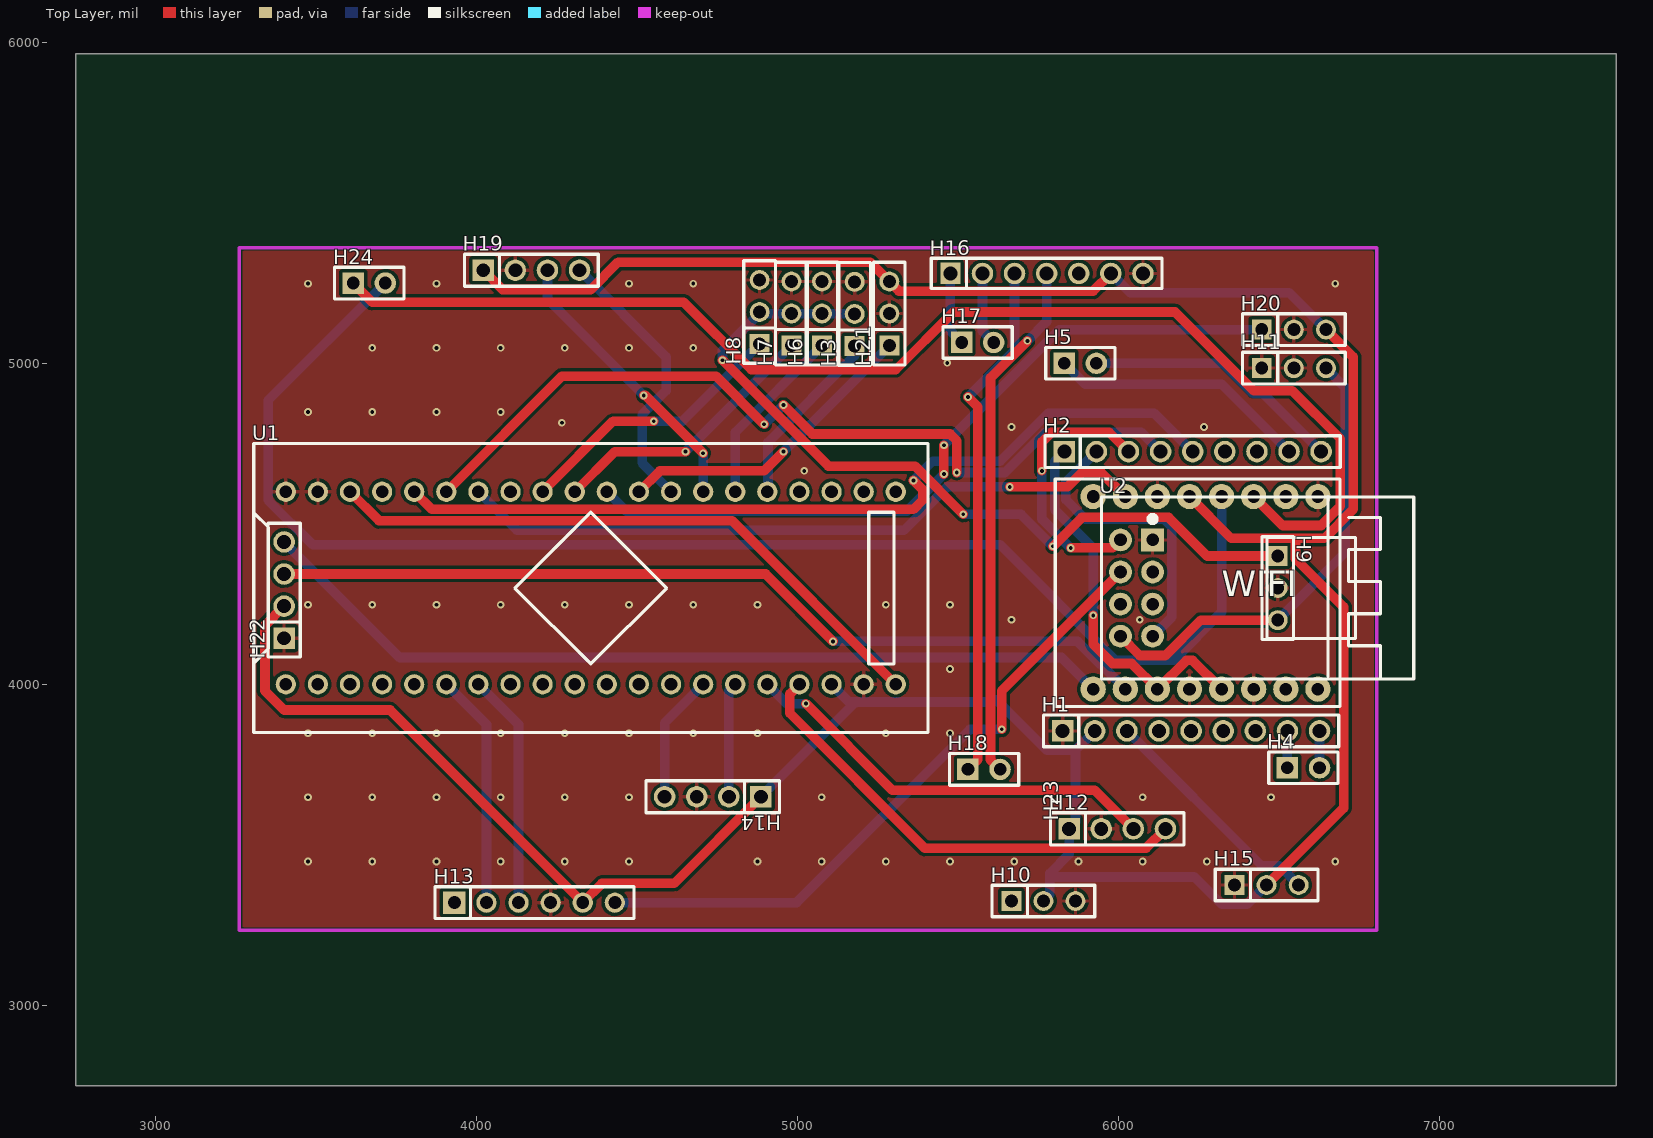
[diagram p0: Top Layer view]
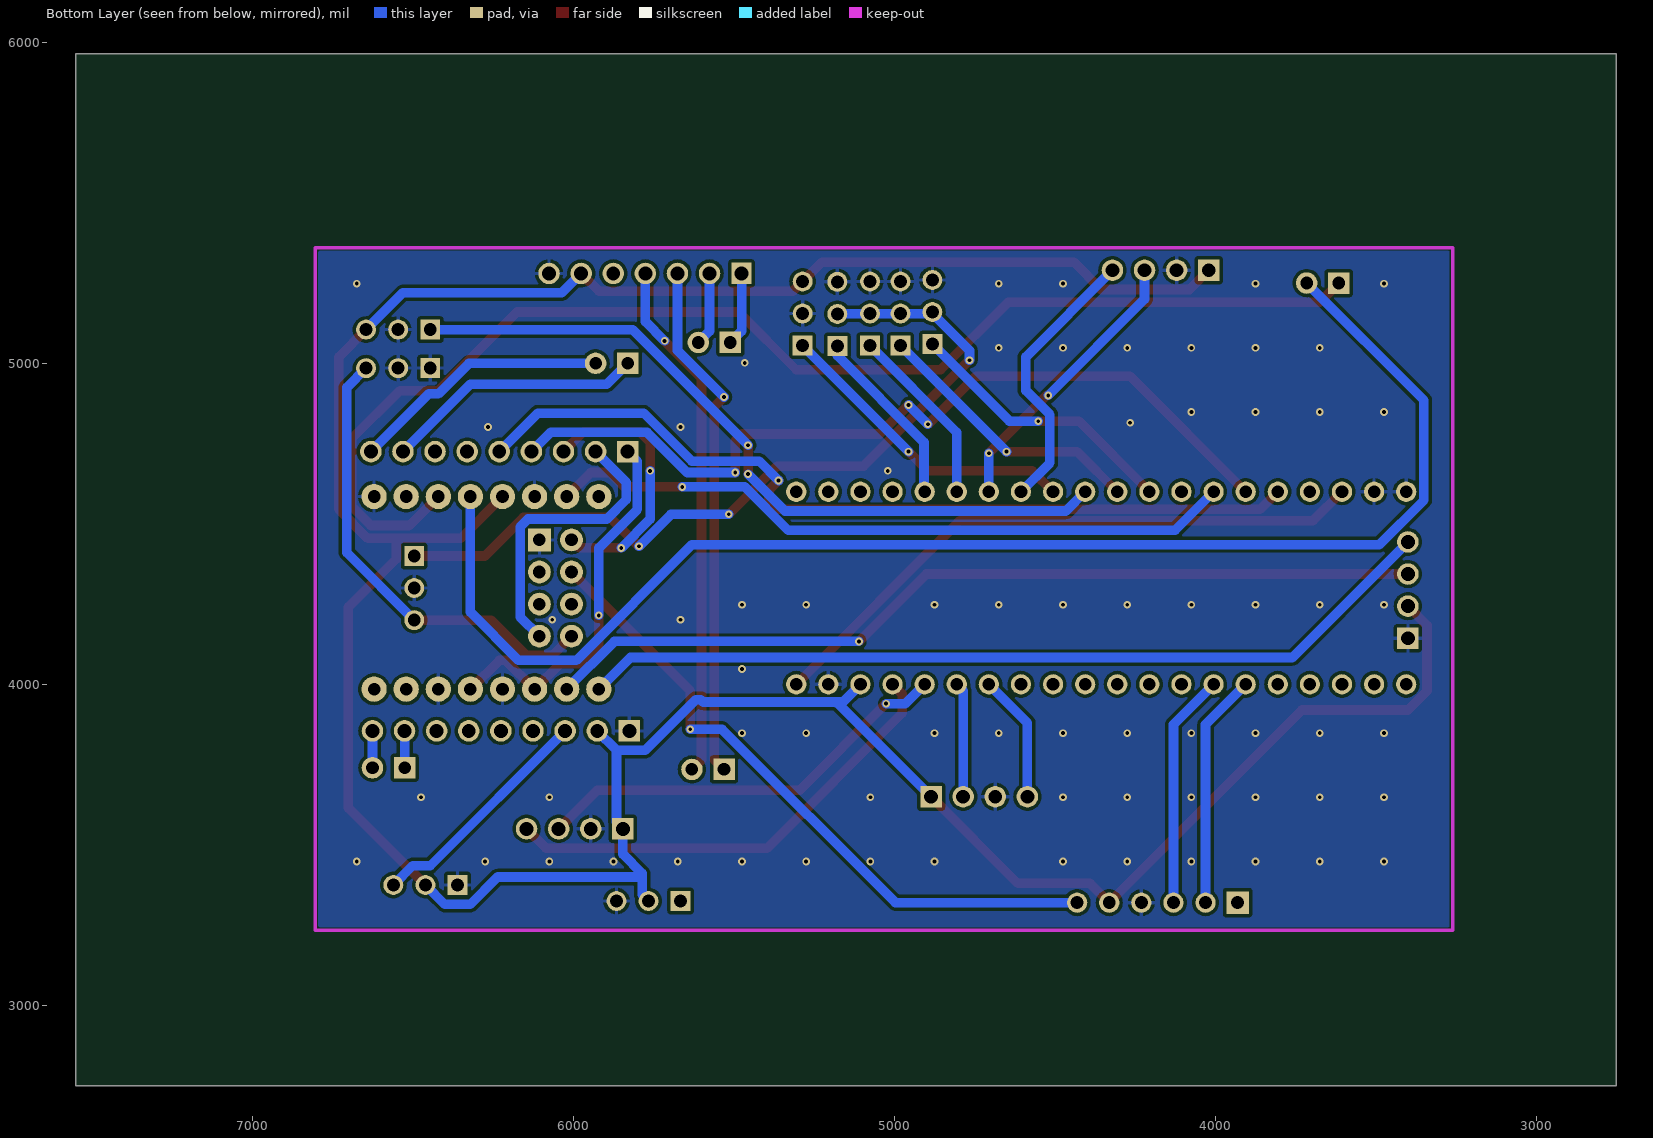
[diagram p1: Bottom Layer view, seen from below]
# Altium PCB MISC49865.pcbdoc
Units mil, origin at the board's own origin, x right, y up, seen from the top; angles counter-clockwise.
Board outline 4800 x 3215 mil, 2 copper layers (Top Layer, Bottom Layer), stack 62.206 mil thick; 26 components, 71 nets, 151 pads, 90 vias.

## Layer stack, top to bottom
Top Solder Mask Layer: solder mask 0.394, Dk 3.3
Top Layer: signal copper 1.379
Dielectric1: surface 59.449, FR4, Dk 4.5
Bottom Layer: signal copper 1.378
Bottom Solder Mask Layer: solder mask 0.394, Dk 3.3

## Board outline
7550,2750 2750,2750 2750,5965 7550,5965

## Design rules (kind name [scope] priority, off if disabled: settings)
BoardOutlineClearance copperThickness2oz_1 [All] p2 off: genericclearance=7.99 ignorepadtopadclearanceinfootprint=FALSE except(0: Arc-SplitContinuation Track-SplitContinuation SMDPad-SplitContinuation THPad-SplitContinuation Via-SplitContinuation Fill-SplitContinuation Region-SplitContinuation Poly-SplitContinuation Text-SplitContinuation Hole-SplitContinuation; 5.98: Arc-CutoutEdge SMDPad-CutoutEdge THPad-CutoutEdge Via-CutoutEdge Fill-CutoutEdge Region-CutoutEdge Text-CutoutEdge; 6.93: Hole-OutlineEdge Hole-CutoutEdge; 10: Poly-OutlineEdge Poly-CutoutEdge; 11.81: Arc-OutlineEdge Track-OutlineEdge SMDPad-OutlineEdge THPad-OutlineEdge Via-OutlineEdge Fill-OutlineEdge Region-OutlineEdge Text-OutlineEdge Track-CutoutEdge)
BoardOutlineClearance copperThickness1oz_1 [All] p4: genericclearance=4.02 ignorepadtopadclearanceinfootprint=FALSE except(0: Arc-SplitContinuation Track-SplitContinuation SMDPad-SplitContinuation THPad-SplitContinuation Via-SplitContinuation Fill-SplitContinuation Region-SplitContinuation Poly-SplitContinuation Text-SplitContinuation Hole-SplitContinuation; 6: SMDPad-CutoutEdge THPad-CutoutEdge Via-CutoutEdge Fill-CutoutEdge Region-CutoutEdge Text-CutoutEdge; 6.93: Hole-OutlineEdge Hole-CutoutEdge; 10: Poly-OutlineEdge Poly-CutoutEdge; 11.8: Arc-OutlineEdge Track-OutlineEdge SMDPad-OutlineEdge THPad-OutlineEdge Via-OutlineEdge Fill-OutlineEdge Region-OutlineEdge Text-OutlineEdge; 11.81: Arc-CutoutEdge Track-CutoutEdge)
Clearance copperThickness2oz [All] p1 off: gap=7.99 ignorepadtopadclearanceinfootprint=FALSE except(5.98: SMDPad-Track SMDPad-SMDPad THPad-Track SMDPad-THPad THPad-THPad Track-Via SMDPad-Via THPad-Via Via-Via Fill-Track Region-Track Fill-SMDPad Region-SMDPad Fill-THPad Region-THPad Fill-Via Region-Via Fill-Fill Fill-Region Region-Region Arc-Track Arc-SMDPad Arc-THPad Arc-Via Fill-Arc Region-Arc Arc-Arc Text-Track SMDPad-Text Text-THPad Text-Via Fill-Text Region-Text Arc-Text Text-Text; 6.93: Hole-Track Hole-SMDPad Hole-THPad Hole-Via Fill-Hole Region-Hole Hole-Arc Hole-Text; 10: Poly-Track Poly-SMDPad Poly-THPad Poly-Via Poly-Fill Poly-Region Poly-Poly Poly-Arc Poly-Text Poly-Hole)
Clearance copperThickness1oz [All] p3: gap=4.02 ignorepadtopadclearanceinfootprint=FALSE except(5.98: SMDPad-Track SMDPad-SMDPad THPad-Track SMDPad-THPad THPad-THPad Track-Via SMDPad-Via THPad-Via Via-Via Fill-Track Region-Track Fill-SMDPad Region-SMDPad Fill-THPad Region-THPad Fill-Via Region-Via Fill-Fill Fill-Region Region-Region; 6: Arc-Track Arc-SMDPad Arc-THPad Arc-Via Fill-Arc Region-Arc Arc-Arc Text-Track SMDPad-Text Text-THPad Text-Via Fill-Text Region-Text Arc-Text Text-Text; 6.93: Hole-Track Hole-SMDPad Hole-THPad Hole-Via Fill-Hole Region-Hole Hole-Arc Hole-Text; 10: Poly-Track Poly-SMDPad Poly-THPad Poly-Via Poly-Fill Poly-Region Poly-Poly Poly-Arc Poly-Text Poly-Hole)
DiffPairsRouting differentialPair [All] p1: maxlimit=6 minlimit=6 mostfreqgap=6 toplayer_minwidth=5 toplayer_prefwidth=10 toplayer_maxwidth=100 toplayer_mingap=6 toplayer_prefgap=6 toplayer_maxgap=6 bottomlayer_minwidth=5 bottomlayer_prefwidth=10 bottomlayer_maxwidth=100 bottomlayer_mingap=6 bottomlayer_prefgap=6 bottomlayer_maxgap=6 maxuncoupledlength=10
HoleToHoleClearance otherClearance [All] p1: gap=11.81 allowstackedmicrovias=TRUE
Length netLength [All] p1: minlimit=0 maxlimit=0
MatchedLengths netLengthTolerance [All] p1: tolerance=1000
PasteMaskExpansion pasteMaskExpansion [All] p1: expansion=0
PlaneConnect innerPlane [All] p1: planeconnectstyle=Relief reliefexpansion=20 reliefentries=4 reliefconductorwidth=10 reliefairgap=10
PolygonConnect copperRegion [All] p1: connectstyle=Relief reliefconductorwidth=10 reliefentries=4 polygonreliefangle="90 Angle" airgapwidth=10 via.connectstyle=Relief via.reliefconductorwidth=10 via.reliefentries=4 via.polygonreliefangle="90 Angle" via.airgapwidth=10
RoutingVias viaSize [All] p1: holewidth=12.01 width=24.02 viastyle="Through Hole" minholewidth=11.81 minwidth=19.68 maxholewidth=248.03 maxwidth=393.7
SolderMaskExpansion solderMaskExpansion [IsVia] p1: expansion=-1000 istentingtop=TRUE
SolderMaskExpansion solderMaskExpansion [All] p2: expansion=2 istentingtop=FALSE
Width copperThickness2oz_2 [All] p1 off: maxlimit=100 minlimit=8 preferedwidth=10
Width copperThickness1oz_2 [All] p2: maxlimit=10 minlimit=10 preferedwidth=10 toplayer_minwidth=30 toplayer_maxwidth=100 toplayer_prefwidth=30 bottomlayer_minwidth=30 bottomlayer_maxwidth=100 bottomlayer_prefwidth=30

## Components (designator, comment, footprint, x,y, rotation, side; value= is the part's Value field where it differs from the comment)
H1 "" HDR-TH_9P-P2.54-V-F-1 6225,3855 r0 top
H2 "" HDR-TH_9P-P2.54-V-F-1 6230,4725 r0 top
H3 "" HDR-TH_3P-P2.54-V-F 5176.94,5153.94 r90 top
H4 "" HDR-TH_2P-P2.54-V-F 6575,3740 r0 top
H5 "" HDR-TH_2P-P2.54-V-F 5880,5000 r0 top
H6 "" HDR-TH_3P-P2.54-V-F 5075,5155 r90 top
H7 "" HDR-TH_3P-P2.54-V-F 4980,5155 r90 top
H8 "" HDR-TH_3P-P2.54-V-F 4880.94,5159.77 r90 top
H9 "" HDR-TH_3P-P2.54-V-F 6495,4300 r270 top
H10 "" HDR-TH_3P-P2.54-V-F 5765,3325 r0 top
H11 "" HDR-TH_3P-P2.54-V-F 6545,4985 r0 top
H12 "" HDR-TH_4P-P2.54-V-F 5995,3550 r0 top
H13 "" HDR-TH_6P-P2.54-V-F 4180,3320 r0 top
H14 "" HDR-TH_4P-P2.54-V-F 4735,3650 r180 top
H15 "" HDR-TH_3P-P2.54-V-F 6460,3375 r0 top
H16 "" HDR-TH_7P-P2.54-V-F 5775,5280 r0 top
H17 "" HDR-TH_2P-P2.54-V-F 5560,5065 r0 top
H18 "" HDR-TH_2P-P2.54-V-F 5580,3735 r0 top
H19 "" HDR-TH_4P-P2.54-V-F 4170,5290 r0 top
H20 "" HDR-TH_3P-P2.54-V-F 6545,5105 r0 top
H21 "" HDR-TH_3P-P2.54-V-F 5285,5155 r90 top
H22 "" HDR-TH_4P-P2.54-V-F 3399.74,4293.7 r90 top
H23 "" ESP32C3MINI 5920,3985 r90 top
H24 "" HDR-TH_2P-P2.54-V-F 3665,5250 r0 top
U1 "STM32F103C8T6-Card" CONN-TH_L53.3-W22.9_STM32F103C8T6-CARD 4355,4300 r0 top
U2 "Ai-Thinker ESP-01S ESP8266" WIFIM-TH_8P-L24.7-W14.4-P2.54 6055,4300 r0 top

## Footprints (in the part's own frame and the unit in brackets; to place one, negate y for a bottom-side part, rotate by r counter-clockwise, add the part's x,y. Pads: shape width x height; smd on the part's side, far side on the other; paste and mask are expansions set on the pad)
CONN-TH_L53.3-W22.9_STM32F103C8T6-CARD [mm]
  round 1.6 hole 1: 1(-24.13,-7.62) 2(-21.59,-7.62) 3(-19.05,-7.62) 4(-16.51,-7.62) 5(-13.97,-7.62) 6(-11.43,-7.62) 7(-8.89,-7.62) 8(-6.35,-7.62) 9(-3.81,-7.62) 10(-1.27,-7.62) 11(1.27,-7.62) 12(3.81,-7.62) 13(6.35,-7.62) 14(8.89,-7.62) 15(11.43,-7.62) 16(13.97,-7.62) 17(16.51,-7.62) 18(19.05,-7.62) 19(21.59,-7.62) 20(24.13,-7.62) 21(24.13,7.62) 22(21.59,7.62) 23(19.05,7.62) 24(16.51,7.62) 25(13.97,7.62) 26(11.43,7.62) 27(8.89,7.62) 28(6.35,7.62) 29(3.81,7.62) 30(1.27,7.62) 31(-1.27,7.62) 32(-3.81,7.62) 33(-6.35,7.62) 34(-8.89,7.62) 35(-11.43,7.62) 36(-13.97,7.62) 37(-16.51,7.62) 38(-19.05,7.62) 39(-21.59,7.62) 40(-24.13,7.62)
  silkscreen extent -26.67,-11.43 26.67,11.43
ESP32C3MINI [mm]
  round 2 hole 1: 1(0,0) 2(0,-2.54) 3(0,-5.08) 4(0,-7.62) 5(0,-10.16) 6(0,-12.7) 7(0,-15.24) 8(0,-17.78) 9(15.24,-17.78) 10(15.24,-15.24) 11(15.24,-12.7) 12(15.24,-10.16) 13(15.24,-7.62) 14(15.24,-5.08) 15(15.24,-2.54) 16(15.24,0)
  silkscreen extent -1.38,-20.75 16.62,3
HDR-TH_2P-P2.54-V-F [mm]
  rect 1.7x1.7 hole 1: 1(-1.27,0)
  round 1.7 hole 1: 2(1.27,0)
  silkscreen extent -2.74,-1.25 2.74,1.25
HDR-TH_3P-P2.54-V-F [mil]
  rect 62x62 hole 40.16: 1(-100,0)
  round 62 hole 40.16: 2(0,0) 3(100,0)
  silkscreen extent -160,-49 160,49
HDR-TH_4P-P2.54-V-F [mm]
  rect 1.7x1.7 hole 1.1: 1(-3.81,0)
  round 1.7 hole 1.1: 2(-1.27,0) 3(1.27,0) 4(3.81,0)
  silkscreen extent -5.29,-1.27 5.29,1.27
HDR-TH_6P-P2.54-V-F [mm]
  rect 1.8x1.8 hole 1.02: 1(-6.35,0)
  round 1.6 hole 1.02: 2(-3.81,0) 3(-1.27,0) 4(1.27,0) 5(3.81,0) 6(6.35,0)
  silkscreen extent -7.87,-1.25 7.87,1.25
HDR-TH_7P-P2.54-V-F [mm]
  rect 1.575x1.7 hole 1.1: 1(-7.62,0)
  round 1.7 hole 1.1: 2(-5.08,0) 3(-2.54,0) 4(0,0) 5(2.54,0) 6(5.08,0) 7(7.62,0)
  silkscreen extent -9.13,-1.2 9.13,1.2
HDR-TH_9P-P2.54-V-F-1 [mm]
  rect 1.7x1.7 hole 1.1: 1(-10.16,0)
  round 1.7 hole 1.1: 2(-7.62,0) 3(-5.08,0) 4(-2.54,0) 5(0,0) 6(2.54,0) 7(5.08,0) 8(7.62,0) 9(10.16,0)
  silkscreen extent -11.68,-1.25 11.68,1.25
WIFIM-TH_8P-L24.7-W14.4-P2.54 [mm]
  rect 1.8x1.8 hole 1 paste+0 mask+0.05: 1(1.27,3.81)
  round 1.8 hole 1 paste+0 mask+0.05: 2(1.27,1.27) 3(1.27,-1.27) 4(1.27,-3.81) 5(-1.27,3.81) 6(-1.27,1.27) 7(-1.27,-1.27) 8(-1.27,-3.81)
  silkscreen extent -2.77,-7.19 21.93,7.24

## Via types
v1: diameter 24.02, hole 12, Top Layer to Bottom Layer, 90 vias

## Nets (pads, with @x,y where several pads share a name; then routed paths per layer and width w, separated by ;. In a path a pad name is that pad's centre, name@x,y a point inside that pad or via, vN(x,y) a via of type N, cw(c..) or ccw(c..) an arc to the next point about the centre after c; other vN are vias at no path point)
3.3V: U1.20 U1.38 | length 1948.5
  Top Layer w30: U1.38 3695,4510 4795,4510 U1.20
3V3: H2.1 H23.3 H23.5 | length 1194.7
  Top Layer w30: v1(5920,4215) 5920,4125 5980,4065 6040,4065 H23.3 6210,4075 6230,4075 H23.5
  Bottom Layer w30: H2.1 5800,4695 5800,4545 5920,4425 v1(5920,4215)
$1N17145: H1.9 H4.2 | length 115
  Bottom Layer w30: H4.2 H1.9
$1N17146: H1.8 H4.1 | length 115
  Bottom Layer w30: H4.1 H1.8
$1N17147: H2.9 H5.2 | length 813.9
  Bottom Layer w30: H5.2 6325,5000 6420,4905 6450,4905 H2.9
$1N17148: H2.8 H5.1 | length 813.9
  Bottom Layer w30: H5.1 5895,4935 6320,4935 H2.8
$1N17189: H16.1 H17.1 | length 229.5
  Bottom Layer w30: H16.1 5475,5099.99 H17.1
$1N17190: H16.2 H17.2 | length 229.5
  Bottom Layer w30: H16.2 5575,5099.99 H17.2
$1N17191: H16.3 H18.1 | length 1629.9
  Top Layer w30: H18.1 5560,3765 5560,4865 v1(5530,4895)
  Bottom Layer w30: v1(5530,4895) 5675,5040 H16.3
$1N17192: H16.4 H18.2 | length 1629.9
  Top Layer w30: H18.2 5600,3765 5600,4955 v1(5715,5070)
  Bottom Layer w30: v1(5715,5070) 5775,5130 H16.4
$1N17229: H23.11 H24.1 | length 3967.1
  Top Layer w30: H24.1 3675,5190 4645,5190 4855,4980 5305,4980 5485,5160 6175,5160 6420,4915 6540,4915 6690,4765 6690,4555 6630,4495 6510,4495 H23.11
$1N17230: H23.12 H24.2 | length 4426.3
  Bottom Layer w30: H24.2 3350.01,4885.01 3350.01,4573.52 3488.52,4435 5630,4435 5990,4075 6170,4075 6320,4225 H23.12
+5V: H1.2 H10.2 H12.1 H13.5 H14.1 H15.2 H16.6 H19.1 H20.3 H21.3 H22.2 H23.13 U1.18 | length 10096.6
  Top Layer w30: H22.2 3340,4183.97 3340,3980 3400,3920 3730,3920 H13.5 4390,3380 4615,3380 H14.1 ; H19.1 4080,5230 4355,5230 4440,5315 5225,5315 H21.3 5315,5225 5920,5225 H16.6 ; H23.13 6350,4455 6550,4455 ; H15.2 6700,3615 6700,4241.22 6550,4391.22 6550,4455 ; H20.3 6730,5020 6730,4545 6640,4455 6550,4455
  Bottom Layer w30: H14.1 5175,3940 5175,3945 ; U1.18 5160,3945 5175,3945 ; H10.2 5785,3345 5785,3400 ; H1.2 5865,3795 ; H16.6 6035,5220 6530,5220 H20.3 ; H15.2 6400,3315 6320,3315 6235,3400 5785,3400 ; 5175,3945 5595,3945 5602.5,3952.5 5617.5,3952.5 5775,3795 5865,3795 ; 5785,3400 5785,3411.26 5845,3471.26 H12.1 5865,3570 5865,3795
BAT_3.7V: H9.3 H11.3 U2.8 | length 1457.3
  Top Layer w30: U2.8 6065,4090 6145,4090 6255,4200 H9.3
  Bottom Layer w30: H9.3 6705,4410 6705,4925 H11.3
EN: H13.6 U2.6 | length 2071.9
  Top Layer w30: v1(5635,3860) 5635,3980 U2.6
  Bottom Layer w30: H13.6 4996.22,3320 5536.22,3860 v1(5635,3860)
GND: H1.1 H3.3 H6.3 H7.3 H8.3 H9.2 H10.3 H11.1 H11.2 H12.2 H13.4 H14.3 H15.1 H16.7 H19.2 H20.2 H21.2 H22.1 H23.4 H23.6 H23.9 H23.14 U1.19 U1.39 U1.40 U2.1
  other v1: 3474.1,3448.12 3674.1,3448.12 3874.1,3448.12 4074.1,3448.12 4274.1,3448.12 4474.1,3448.12 4874.1,3448.12 5074.1,3448.12 5274.1,3448.12 5474.1,3448.12 5674.1,3448.12 5874.1,3448.12 6074.1,3448.12 6274.1,3448.12 6674.1,3448.12 3474.1,3648.12 3674.1,3648.12 3874.1,3648.12 4074.1,3648.12 4274.1,3648.12 4474.1,3648.12 5074.1,3648.12 6074.1,3648.12 6474.1,3648.12 3474.1,3848.12 3674.1,3848.12 3874.1,3848.12 4074.1,3848.12 4274.1,3848.12 4474.1,3848.12 4674.1,3848.12 4874.1,3848.12 5274.1,3848.12 5474.1,3848.12 5474.1,4048.12 5665.25,4201.38 6065.25,4201.38 3474.1,4248.12 3674.1,4248.12 3874.1,4248.12 4074.1,4248.12 4274.1,4248.12 4474.1,4248.12 4674.1,4248.12 4874.1,4248.12 5274.1,4248.12 5474.1,4248.12 5020,4665 5665.25,4801.38 6265.25,4801.38 4265,4815 3474.1,4848.12 3674.1,4848.12 3874.1,4848.12 4074.1,4848.12 5465.25,5001.38 3674.1,5048.12 3874.1,5048.12 4074.1,5048.12 4274.1,5048.12 4474.1,5048.12 4674.1,5048.12 3474.1,5248.12 3874.1,5248.12 4474.1,5248.12 4674.1,5248.12 6674.1,5248.12
IO0: U2.3
IO2: U2.2
MOTOR_+5V: H3.2 H6.2 H7.2 H8.2 H9.1 | length 2555
  Top Layer w30: v1(4765.23,5009.77) 5095.23,4679.77 5365.23,4679.77 v1(5515.23,4529.77) ; v1(5795,4430) 5885,4520 6155,4520 6275,4400 H9.1
  Bottom Layer w30: v1(4765.23,5009.77) 4765.23,5039.77 H8.2@4885.23,5159.77 ; H8.2 H8.2@4885.23,5159.77 ; H3.2 5076.06,5153.94 H6.2 H7.2 4890,5155 H8.2@4885.23,5159.77 ; v1(5515.23,4529.77) 5695.23,4529.77 v1(5795,4430)
MUTE: H1.7
NRST: U1.37
PA0: H3.1 U1.25 | length 566.6
  Bottom Layer w30: U1.25 4906.94,4601.94 4906.94,4753.94 5176.94,5023.94 H3.1
PA0/: H2.7
PA1: H6.1 U1.26 | length 566.8
  Bottom Layer w30: U1.26 4805,4785.01 H6.1
PA1/: H2.6
PA2: H19.3 U1.27 | length 893.8
  Top Layer w30: v1(4520,4900) 4525,4900 v1(4705,4720)
  Bottom Layer w30: H19.3 4220,5200 v1(4520,4900) ; U1.27 v1(4705,4720)
PA3: H19.4 U1.28 | length 870.2
  Bottom Layer w30: H19.4 4590,5020 4590,4915 4515,4840 4515,4690 U1.28
PA4: H21.1 U1.29 | length 968.5
  Top Layer w30: U1.29 4570.01,4665 4895,4665 v1(4955,4725)
  Bottom Layer w30: v1(4955,4725) H21.1
PA4/: H1.6
PA5: H20.1 U1.30 | length 2351.6
  Top Layer w30: v1(5455,4655) v1(5455,4745)
  Bottom Layer w30: U1.30 4465,4540 5340,4540 v1(5455,4655) ; v1(5455,4745) 5815,5105 H20.1
PA5/: H2.3 U2.5 | length 839.9
  Top Layer w30: v1(5760,4665) 5760,4755 5790,4785 5970,4785 H2.3 ; v1(5850,4425) 5980,4425 U2.5
  Bottom Layer w30: v1(5760,4665) 5760,4515 v1(5850,4425)
PA6: H7.1 U1.31 | length 863.5
  Top Layer w30: U1.31 4430,4725 v1(4650,4725)
  Bottom Layer w30: v1(4650,4725) H7.1
PA6/: H2.2 U2.4 | length 919.8
  Bottom Layer w30: H2.2 5835,4630 5835,4575 5895,4515 6140.68,4515 6165,4490.68 6165,4210 U2.4
PA7: H8.1 U1.32 | length 866.4
  Top Layer w30: U1.32 4424.77,4819.77 v1(4550.94,4819.77)
  Bottom Layer w30: v1(4550.94,4819.77) 4640.94,4819.77 H8.1
PA8: U1.5
PA9: H13.2 U1.6 | length 731.8
  Bottom Layer w30: U1.6 4030,3875 H13.2
PA10: H13.3 U1.7 | length 731.8
  Bottom Layer w30: U1.7 4130,3875 H13.3
PA11: U1.8
PA12: U1.9
PA15: U1.10
PB0: U1.33
PB1: H23.15 U1.34 | length 2170.3
  Top Layer w30: v1(5660,4615) 5840,4615 5885,4660 5945,4660 H23.15
  Bottom Layer w30: U1.34 4125,4480 5330,4480 5465,4615 v1(5660,4615)
PB3: U1.11
PB4: U1.12
PB5: U1.13
PB5/: H1.3 H15.3 | length 733.8
  Bottom Layer w30: H1.3 6445,3435 6500,3435 H15.3
PB6: H14.4 U1.14 | length 399.7
  Bottom Layer w30: H14.4 4585,3880 U1.14
PB6/: H1.4
PB7: H14.2 U1.15 | length 358.3
  Bottom Layer w30: H14.2 4785,3980 U1.15
PB8: H12.3 U1.16 | length 1326.4
  Top Layer w30: v1(5025,3940) 5295,3670 5925,3670 H12.3
  Bottom Layer w30: U1.16 4965,3940 v1(5025,3940)
PB9: H12.4 U1.17 | length 1471.2
  Top Layer w30: U1.17 4975,3970 4975,3910 5395,3490 6085,3490 H12.4
PB10: H2.4 U1.35 | length 2682.9
  Top Layer w30: U1.35 4265,4960 4745,4960 v1(4895,4810) ; v1(4955,4870) 5045,4780 5474.37,4780 5495,4759.37 v1(5495,4660)
  Bottom Layer w30: v1(4895,4810) v1(4955,4870) ; v1(5495,4660) 5645,4660 5770,4785 6070,4785 H2.4
PB11: H2.5 U1.36 | length 2699.3
  Top Layer w30: U1.36 3860.01,4545 5360,4545 5390,4575 5390,4605 v1(5360,4635)
  Bottom Layer w30: v1(5360,4635) 5420,4695 5630,4695 5780,4845 6110,4845 H2.5
PB12: U1.1
PB13: U1.2
PB14: U1.3
PB15: U1.4
PC4/: H1.5
PC13: U1.22
PC14: U1.23
PC15: U1.24
RST: U2.7
SCK: H22.3 H23.2 | length 2768.8
  Top Layer w30: H22.3 4899.73,4343.7 v1(5109.73,4133.7)
  Bottom Layer w30: v1(5109.73,4133.7) 5871.3,4133.7 H23.2
SDA: H22.4 H23.1 | length 2710.3
  Bottom Layer w30: H22.4 3759.73,4083.7 5821.3,4083.7 H23.1
STATE: H13.1
TYPE-C_+5V: H10.1
U1RXD: H23.7
U1TXD: H23.8
VBAT: H16.5
VBT: U1.21
VSYS: H23.10
pads on no net: H23.16

## Polygon pours and split planes (outlines as drawn)
GND on Top Layer (solid, remove dead copper, pour order 0): 3000,5615 3000,3000 7300,3000 7300,5615
GND on Bottom Layer (solid, remove dead copper, pour order 2): 3110,5715 3110,3040 7110,3040 7110,5715

## Keep-outs
Board Outline Layer:
  lines w10: 3260,3234.02 3260,5360 6803.31,5360 6803.31,3234.02 3260,3234.02